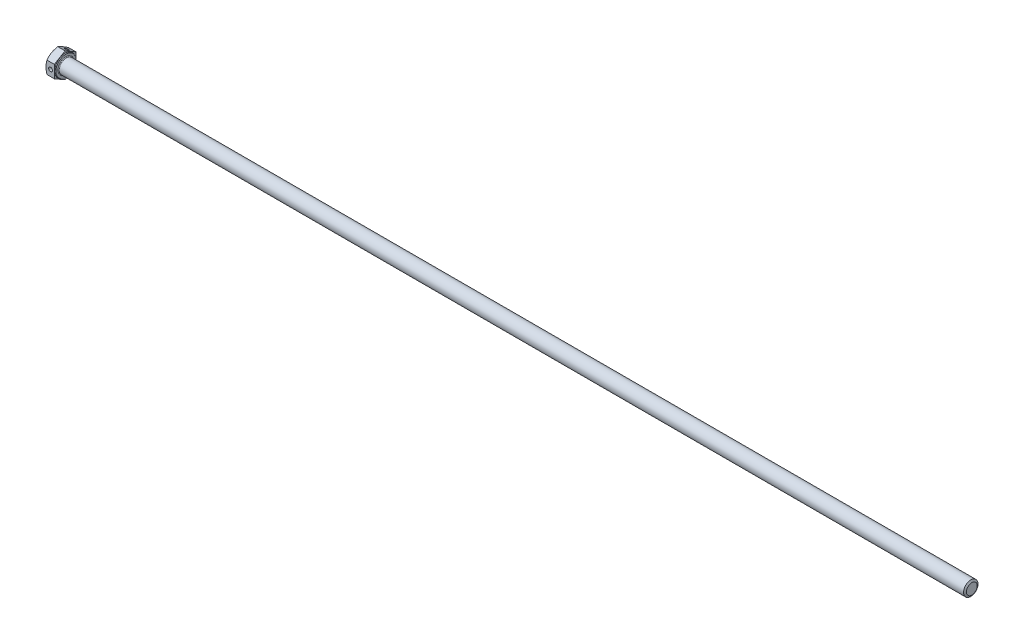
SolidWorks part; units mm, degrees
ref_plane "前视" through (0, 0, 0) normal (0, 0, 1) x (1, 0, 0)
ref_plane "上视" through (0, 0, 0) normal (0, 1, 0) x (1, 0, 0)
ref_plane "右视" through (0, 0, 0) normal (1, 0, 0) x (0, 0, -1)
sketch "草图1" plane through (0, 0, 0) normal (1, 0, 0) x (0, 0, -1)
  line L0 (9, 5.1962) -> (9, -5.1962)
  line L1 (-9, 5.1962) -> (-9, -5.1962)
  line L2 (9, -5.1962) -> (0, -10.3923)
  line L3 (0, -10.3923) -> (-9, -5.1962)
  line L4 (9, 5.1962) -> (0, 10.3923)
  line L5 (0, 10.3923) -> (-9, 5.1962)
  circle A0 centre (0, 0) radius 10.015 construction
  dimension "e" = 20.03
  dimension "s" = 18
  dimension "D2" = 120
  dimension "D3" = 9
  dimension "D4" = 9
  dimension "D5" = 9
extrude "基体-拉伸" add sketch "草图1" along normal blind 7.5
sketch "草图2" plane through (0, 0, 0) normal (0, 0, 1) x (1, 0, 0)
  line L0 (0, 5.1962) -> (0, -5.1962) construction
  line L1 (0, 0) -> (760.5, 0)
  line L2 (0, 0) -> (0, 6)
  line L3 (0, 6) -> (730.5, 6)
  line L4 (760.5, 0) -> (760.5, 4.4845)
  line L5 (7.5, 10.3923) -> (7.5, 5.1962) construction
  line L7 (0, 0) -> (96.52, 0) construction
  line L8 (760.5, -4.4845) -> (730.5, -6) construction
  line L9 (0, -6) -> (730.5, -6) construction
  line L10 (9.25, 6) -> (9.25, 0) construction
  line L11 (730.5, 6) -> (730.5, 0) construction
  line L12 (7.5, 5.1962) -> (7.5, -5.1962) construction
  line L13 (730.5, 6) -> (760.5, 6)
  line L14 (760.5, 6) -> (760.5, 4.4845)
  dimension "l" = 753
  dimension "d" = 12
  dimension "Minor_dia" = 8.969
  dimension "p" = 1.75
  dimension "b" = 30
revolve "凸台-旋转1" add sketch "草图2" angle 360 about L7
cosmetic thread "螺旋线1" parameters "Thread_length"=30, "Thread_minor"=8.969
sketch "草图3" plane through (0, 0, 0) normal (0, 0, 1) x (1, 0, 0)
  line L0 (0, 9) -> (3.6906, 15.3923)
  line L1 (0, 10.3923) -> (0, 5.1962) construction
  line L2 (3.6906, 15.3923) -> (3.6906, 20.3923)
  line L3 (3.6906, 20.3923) -> (-10, 20.3923)
  line L4 (-10, 20.3923) -> (-10, 9)
  line L5 (-10, 9) -> (0, 9)
  line L6 (0, 0) -> (99.06, 0) construction
  line L7 (7.5, 10.3923) -> (0, 10.3923) construction
  dimension "D1" = 9
  dimension "D2" = 5
  dimension "D3" = 10
  dimension "D4" = 5
  dimension "Head_ch_ang" = 30
revolve "切除-旋转1" cut sketch "草图3" angle 360 about L6
sketch "草图5" plane through (0, 0, 0) normal (0, 0, 1) x (1, 0, 0)
  line L0 (0, 0) -> (73.6758, 0) construction
  line L2 (7.5, 0) -> (7.5, 8.315) construction
  line L3 (7.5, -6) -> (7.5, 6) construction
  line L4 (7.5, 8.315) -> (6.9, 8.6614)
  line L5 (6.9, 8.6614) -> (6.9, 10.3923)
  line L6 (7.5, 10.3923) -> (0.8038, 10.3923) construction
  line L10 (6.9, 10.3923) -> (7.5, 10.3923)
  line L11 (7.5, 10.3923) -> (7.5, 8.315)
  dimension "D1" = 120
  dimension "dw" = 16.63
  dimension "c" = 0.6
revolve "切除-旋转5" cut sketch "草图5" angle 360 about L0
fillet "圆角" radius 0.6 1 edges at (7.5, 0, -6)
sketch "草图6" plane through (0, 0, 0) normal (0, 0, 1) x (1, 0, 0)
  line L0 (0, 0) -> (760.5, 0) construction
  line L1 (760.5, -6) -> (760.5, 6) construction
  line L2 (760.5, 0) -> (760.5, 6) construction
  line L4 (759.625, 6) -> (761.375, 6)
  line L5 (759.625, 6) -> (760.5, 4.4845)
  line L6 (760.5, 4.4845) -> (761.375, 6)
  dimension "D1" = 1.75
revolve "切除-旋转4" cut sketch "草图6" angle 360 about L0
pattern_linear "阵列(线性)1" [suppressed]
sketch "草图7" plane through (0, 0, 0) normal (0, 0, 1) x (1, 0, 0)
  line L0 (0, 0) -> (96.52, 0) construction
  line L3 (7.5, 5.1962) -> (7.5, -5.1962) construction
  circle A0 centre (3.8, 0) radius 1.6
  dimension "d1" = 3.2
  dimension "h" = 3.7
extrude "切除-拉伸1" cut sketch "草图7" against normal through all and the other way through all
pattern_circular "阵列(圆周)1" count 2 every 60 about axis through (0, 0, 0) along (1, 0, 0) of "切除-拉伸1"
